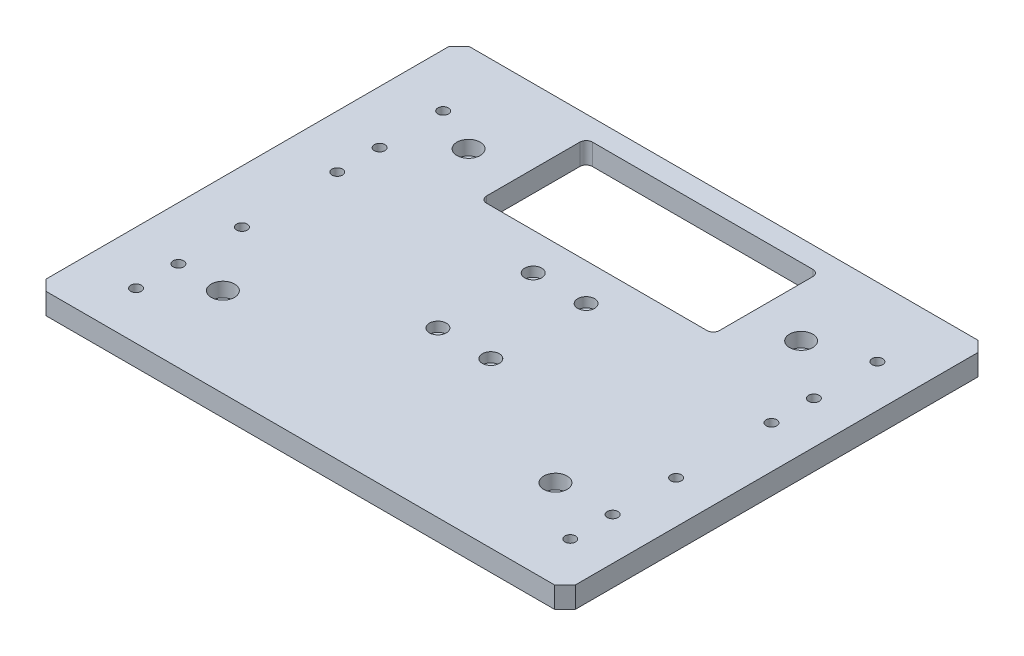
from build123d import *

# Parameters (mm, degrees)
SKETCH1_W                                            = 250
SKETCH1_H                                            = 200
BOSS_EXTRUDE1_DEPTH                                  = 10
M6_TAPPED_HOLE1_D                                    = 5
M6_TAPPED_HOLE1_DEPTH                                = 17
M6_TAPPED_HOLE1_TIP                                  = 1.502151548
SKETCH6_W                                            = 110
SKETCH6_H                                            = 50
CUT_EXTRUDE2_DEPTH                                   = 161.390149323
FILLET1_R                                            = 3
CHAMFER1_SIZE                                        = 5
CBORE_FOR_M6_HEXAGON_SOCKET_HEAD_CAP_SCR_D           = 6.6
CBORE_FOR_M6_HEXAGON_SOCKET_HEAD_CAP_SCR_CBORE_D     = 11
CBORE_FOR_M6_HEXAGON_SOCKET_HEAD_CAP_SCR_CBORE_DEPTH = 6.8
CBORE_FOR_M4_HEXAGON_SOCKET_HEAD_CAP_SCR_D           = 4.5
CBORE_FOR_M4_HEXAGON_SOCKET_HEAD_CAP_SCR_CBORE_D     = 8
CBORE_FOR_M4_HEXAGON_SOCKET_HEAD_CAP_SCR_CBORE_DEPTH = 4.6


with BuildPart() as part:
    # Sketch1 → Boss-Extrude1 (new body)
    with BuildSketch(Plane(origin=(0, 0, 0), x_dir=(1, 0, 0), z_dir=(0, 1, 0))):
        Rectangle(SKETCH1_W, SKETCH1_H)
    extrude(amount=BOSS_EXTRUDE1_DEPTH)

    # M6 Tapped Hole1
    with Locations(Plane(origin=(0, 10, 0), x_dir=(1, 0, 0), z_dir=(0, 1, 0))):
        with Locations((105, -77.5), (-100, -77.5), (-100, 17.5), (105, 17.5), (-100, 37.5), (-100, 67.5), (105, 37.5), (105, 67.5), (-100, -57.5), (-100, -27.5), (105, -57.5), (105, -27.5)):
            Hole(M6_TAPPED_HOLE1_D / 2, depth=M6_TAPPED_HOLE1_DEPTH)
            with Locations((0, 0, -(M6_TAPPED_HOLE1_DEPTH + M6_TAPPED_HOLE1_TIP / 2))):  # 118° drill point
                Cone(0, M6_TAPPED_HOLE1_D / 2, M6_TAPPED_HOLE1_TIP, mode=Mode.SUBTRACT)

    # Sketch6 → Cut-Extrude2 (cut, through all)
    with BuildSketch(Plane(origin=(0, 10, 0), x_dir=(1, 0, 0), z_dir=(0, 1, 0))):
        with Locations((0, 65)):
            Rectangle(SKETCH6_W, SKETCH6_H)
    extrude(amount=-CUT_EXTRUDE2_DEPTH, mode=Mode.SUBTRACT)

    # Fillet1
    fillet1_edges = [part.edges().sort_by_distance(p)[0] for p in [
        (-55, 5, -40),
        (-55, 5, -90),
        (55, 5, -90),
        (55, 5, -40),
    ]]
    fillet(fillet1_edges, radius=FILLET1_R)

    # Chamfer1
    chamfer1_edges = [part.edges().sort_by_distance(p)[0] for p in [
        (125, 5, 100),
        (-125, 5, 100),
        (-125, 5, -100),
        (125, 5, -100),
    ]]
    chamfer(chamfer1_edges, length=CHAMFER1_SIZE)

    # CBORE for M6 Hexagon socket head cap screws1 (through all)
    with Locations(Plane(origin=(0, 10, 0), x_dir=(1, 0, 0), z_dir=(0, 1, 0))):
        with Locations((-78.5, 58), (78.5, 58), (78.5, -58), (-78.5, -58)):
            CounterBoreHole(CBORE_FOR_M6_HEXAGON_SOCKET_HEAD_CAP_SCR_D / 2, CBORE_FOR_M6_HEXAGON_SOCKET_HEAD_CAP_SCR_CBORE_D / 2, CBORE_FOR_M6_HEXAGON_SOCKET_HEAD_CAP_SCR_CBORE_DEPTH)

    # CBORE for M4 Hexagon socket head cap screws1 (through all)
    with Locations(Plane(origin=(0, 10, 0), x_dir=(1, 0, 0), z_dir=(0, 1, 0))):
        with Locations((-12.5, 22.5), (12.5, 22.5), (12.5, -22.5), (-12.5, -22.5)):
            CounterBoreHole(CBORE_FOR_M4_HEXAGON_SOCKET_HEAD_CAP_SCR_D / 2, CBORE_FOR_M4_HEXAGON_SOCKET_HEAD_CAP_SCR_CBORE_D / 2, CBORE_FOR_M4_HEXAGON_SOCKET_HEAD_CAP_SCR_CBORE_DEPTH)


solid = part.part
